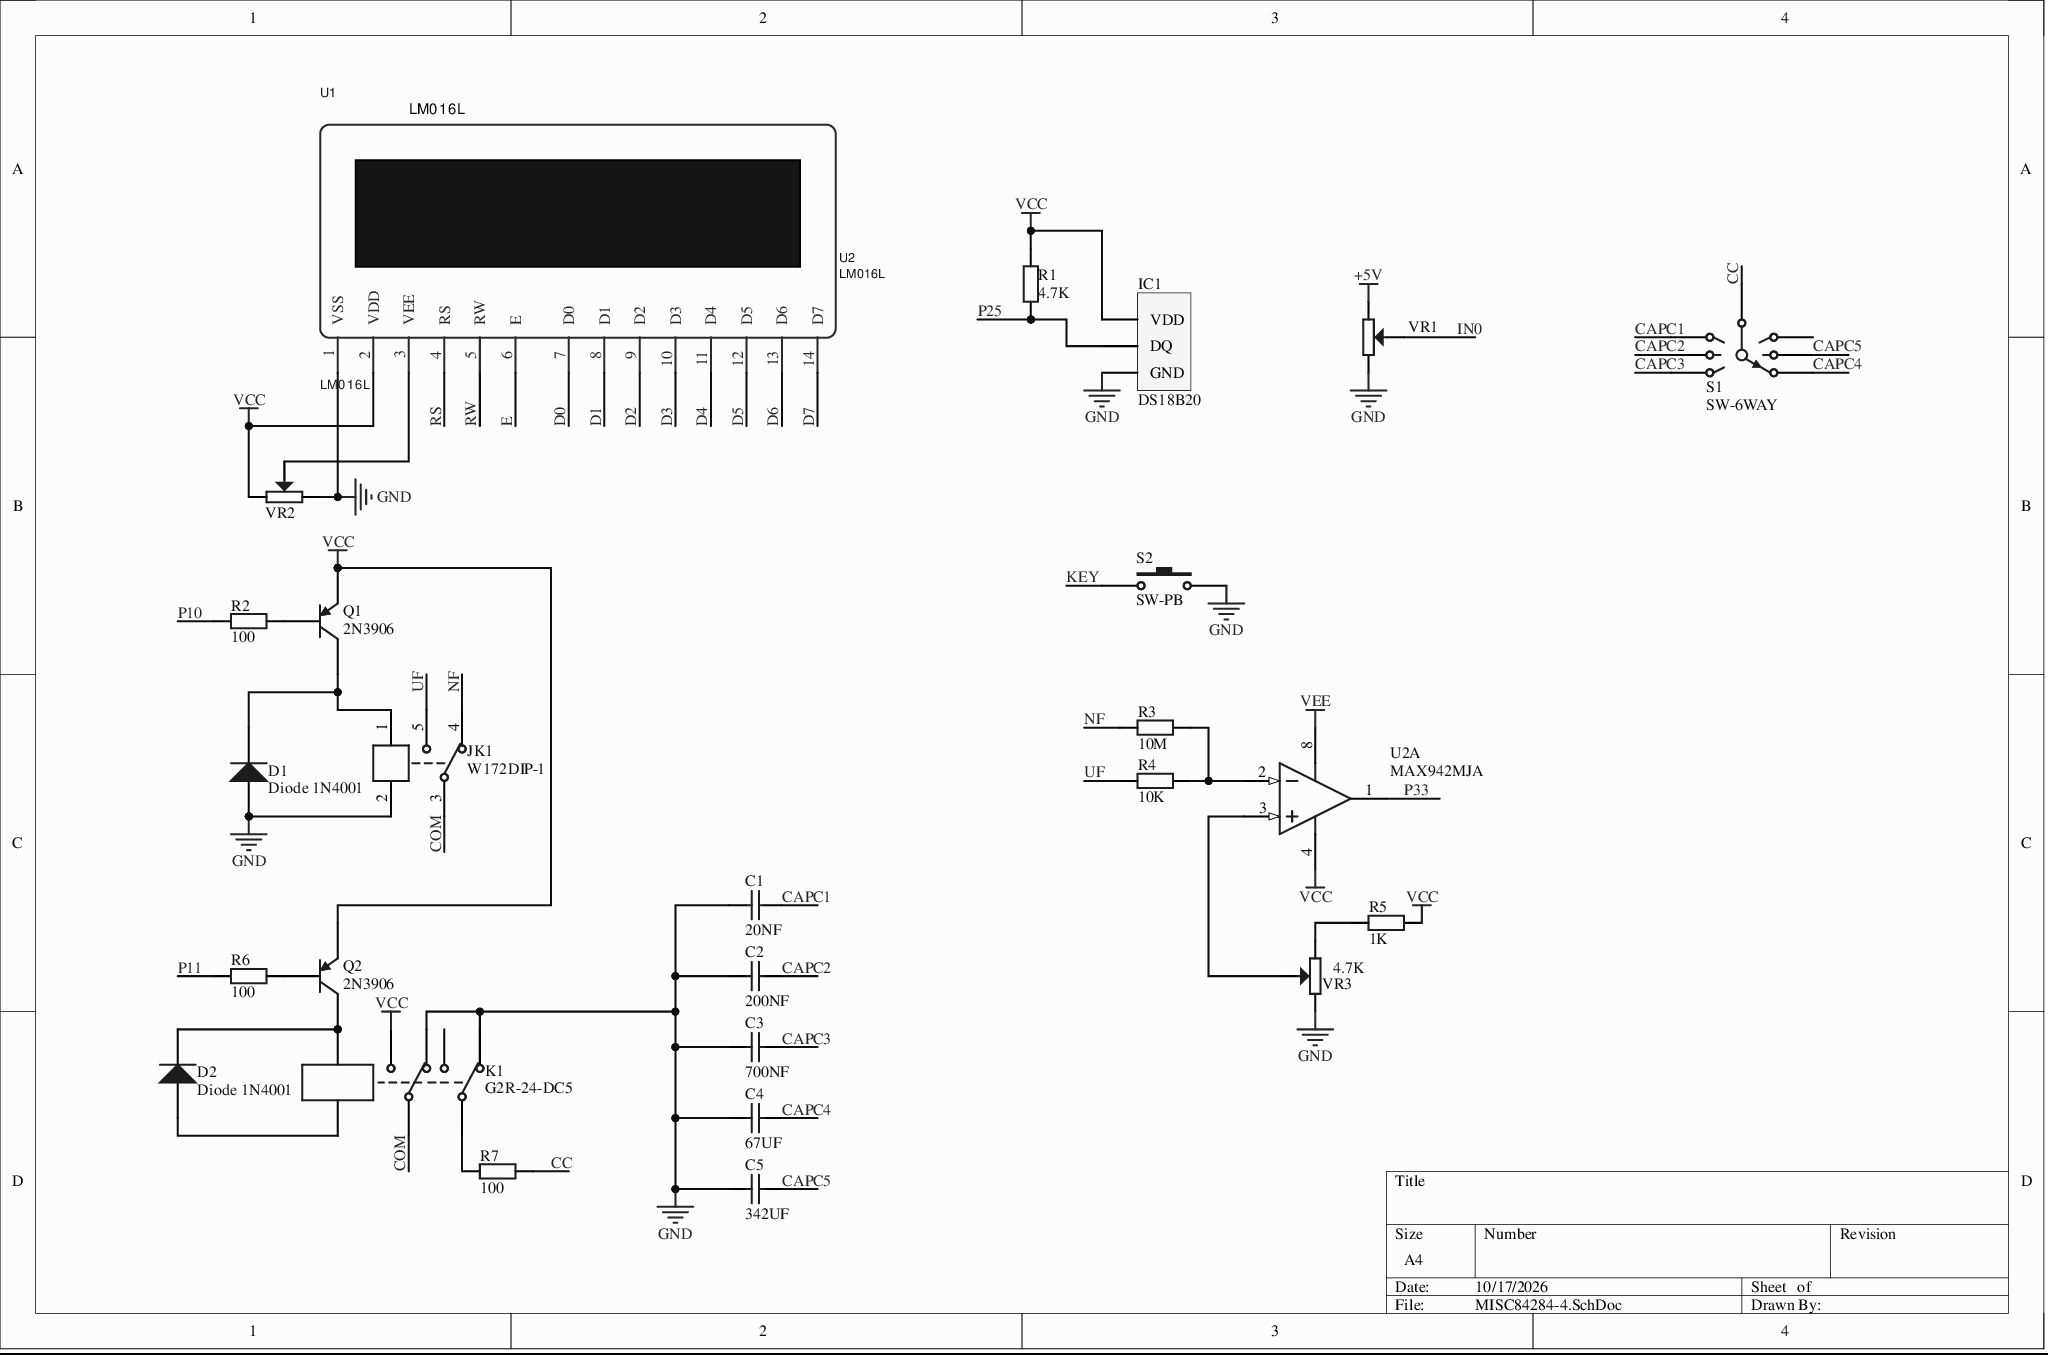
[diagram p0: MISC84284-4.SchDoc]
# Altium project MISC84284-2.PrjPcb
2 sheets, 40 parts. Net scope: global (net labels, ports and power ports of the same name join across sheets).
Board file: MISC84284.PcbDoc
Sheets:
  MISC84284-4.SchDoc
  MISC84284-5.SchDoc

## Sheet MISC84284-4.SchDoc
size A4

### Parts
C1  20NF  [RAD-0.2]
C2  200NF  [RAD-0.2]
C3  700NF  [RAD-0.2]
C4  67UF  [RAD-0.2]
C5  342UF  [RAD-0.2]
D1  Diode 1N4001  [DO-41]
D2  Diode 1N4001  [DO-41]
IC1  DS18B20  [HDR1X3]
JK1  W172DIP-1  [SRD-C_BK]
K1  G2R-24-DC5  [DIP-P8]
Q1  2N3906  [TO-92A]
Q2  2N3906  [TO-92A]
R1  4.7K  [AXIAL-0.4]
R2  100  [AXIAL-0.4]
R3  10M  [AXIAL-0.4]
R4  10K  [AXIAL-0.4]
R5  1K  [AXIAL-0.4]
R6  100  [AXIAL-0.4]
R7  100  [AXIAL-0.4]
S1  SW-6WAY  [SW-7]
S2  SW-PB  [SPST-2]
U1  LM016L  [LM016L]
U2  MAX942MJA  [JA8]  (part A of 2)
VR1  RESVR  [3296W]  (value not drawn)
VR2  RESVR  [3296W]  (value not drawn)
VR3  4.7K  [3296W]

### Nets
+5V: VR1.1
GND: C1.1 C2.1 C3.1 C4.1 C5.1 D1.1(A) IC1.1(GND) JK1.2 K1.2 K1.5 S2.2 U1.1(VSS) VR1.2 VR2.2 VR3.1
VCC: IC1.3(VDD) K1.6 Q1.1(E) Q2.1(E) R1.2 R5.1 U1.2(VDD) U2.4(GND) VR2.1
VEE: U2.8(V+)
CAPC1: C1.2 S1.1
CAPC2: C2.2 S1.2
CAPC3: C3.2 S1.3
CAPC4: C4.2 S1.6
CAPC5: C5.2 S1.5
CC: R7.1 S1.7
COM: JK1.3 K1.4
D0: U1.7(D0)
D1: U1.8(D1)
D2: U1.9(D2)
D3: U1.10(D3)
D4: U1.11(D4)
D5: U1.12(D5)
D6: U1.13(D6)
D7: U1.14(D7)
E: U1.6(E)
IN0: VR1.2
KEY: S2.1
NF: JK1.4 R3.2
P10: R2.2
P11: R6.2
P25: IC1.2(DQ) R1.1
P33: U2.1(OUT)
RS: U1.4(RS)
RW: U1.5(RW)
UF: JK1.5 R4.2
NetD1_2: D1.2(K) JK1.1 Q1.3(C)
NetD2_1: D2.1(A) K1.7
NetD2_2: D2.2(K) K1.8 Q2.3(C)
NetK1_1: K1.1 R7.2
NetQ1_2: Q1.2(B) R2.1
NetQ2_2: Q2.2(B) R6.1
NetR3_1: R3.1 R4.1 U2.2(IN-)
NetR5_2: R5.2 VR3.2
NetU1_3: U1.3(VEE) VR2.2
NetU2_3: U2.3(IN+) VR3.2

Not connected (* = marked no-connect by the designer): K1 3; S1 4

### Library data of the parts
C1-C5 = Cap: Capacitor; Value: 100pF; Published: 8-Jun-2000; LatestRevisionDate: 17-Jul-2002; LatestRevisionNote: Re-released for DXP Platform.; PackageReference: RAD-0.3; PackageDescription: Radial Cap, Thru-Hole; 2 Leads; 0.3 in Pin Spacing; Publisher: Altium Limited
D1 D2 = Diode 1N4001: 1 Amp General Purpose Rectifier; Published: 8-Jun-2000; LatestRevisionDate: 17-Jul-2002; LatestRevisionNote: Re-released for DXP Platform.; DatasheetVersion: 1998; PackageVersion: Aug-1999; PackageReference: DO-41; PackageDescription: Diode, Axial; Body 5.2 x 2.7 mm (LxDia. max), Lead Dia. 0.86 mm (max); Code_JEDEC: DO-204-AL; ComponentLink1Description: Manufacturer Link; ComponentLink2Description: Datasheet; ComponentLink2URL: http://www.fairchildsemi.com/ds/1N%2F1N4001.pdf; Publisher: Altium Limited
IC1 = DS18B20: Digital thermometer; BOM名称: Digital thermometer
JK1 = SRD-S-105D: 5V一组转换; BOM名称: 5V relay
K1 = Relay-DPDT: Dual-Pole Dual-Throw Relay; Published: 24-Mar-1999; LatestRevisionDate: 17-Jul-2002; LatestRevisionNote: Re-released for DXP Platform.; PackageReference: DIP-P8; PackageDescription: Relay; 8 Leads; Publisher: Altium Limited
Q1 Q2 = 2N3906: PNP General Purpose Amplifier; Published: 8-Jun-2000; LatestRevisionDate: 15-Jan-2003; LatestRevisionNote: PCB Footprint 'BCY-W3/D4.7' replaced; DatasheetVersion: 1997; PackageVersion: Sep-1998; PackageReference: TO-92A; PackageDescription: TO, Flat Index; 3 In-Line, Axial Leads; Body Dia. 4.5mm; Leads 0.51 x 0.48 mm (max); ComponentLink1Description: Manufacturer Link; ComponentLink2Description: Datasheet; ComponentLink2URL: http://www.fairchildsemi.com/ds/2N%2F2N3906.pdf; Publisher: Altium Limited
R1-R4 R6 R7 = Res2: Resistor; Value: 1K; Published: 8-Jun-2000; LatestRevisionDate: 17-Jul-2002; LatestRevisionNote: Re-released for DXP Platform.; PackageReference: AXIAL-0.4; PackageDescription: Axial Device, Thru-Hole; 2 Leads; 0.4 in Pin Spacing; Publisher: Altium Limited
R5 = Res2: Resistor; Published: 8-Jun-2000; LatestRevisionDate: 17-Jul-2002; LatestRevisionNote: Re-released for DXP Platform.; PackageReference: AXIAL-0.4; PackageDescription: Axial Device, Thru-Hole; 2 Leads; 0.4 in Pin Spacing; Value: 1K; Publisher: Altium Limited
S1 = SW-6WAY: 6 Way Switch; Published: 24-Mar-1999; LatestRevisionDate: 17-Jul-2002; LatestRevisionNote: Re-released for DXP Platform.; PackageReference: SW-7; PackageDescription: Switch; 7 Leads; Publisher: Altium Limited
S2 = SW-PB: Switch; Published: 24-Mar-1999; LatestRevisionDate: 17-Jul-2002; LatestRevisionNote: Re-released for DXP Platform.; PackageReference: SPST-2; PackageDescription: Switch; 2 Leads; Publisher: Altium Limited
U2 = MAX942MJA: High-speed, Low-power, 3V/5V, Rail-to-Rail Dual-Supply Comparator; Package Information: Latest Revision: 1996; Published: 16-Jan-2001; Revision: 17-Jul-2002: Re-released for DXP Platform.; Datasheet: Latest Revision: Jun-1997; Package Reference: JA8; Publisher: Altium Limited
VR3 = RESVR

## Sheet MISC84284-5.SchDoc
size A4
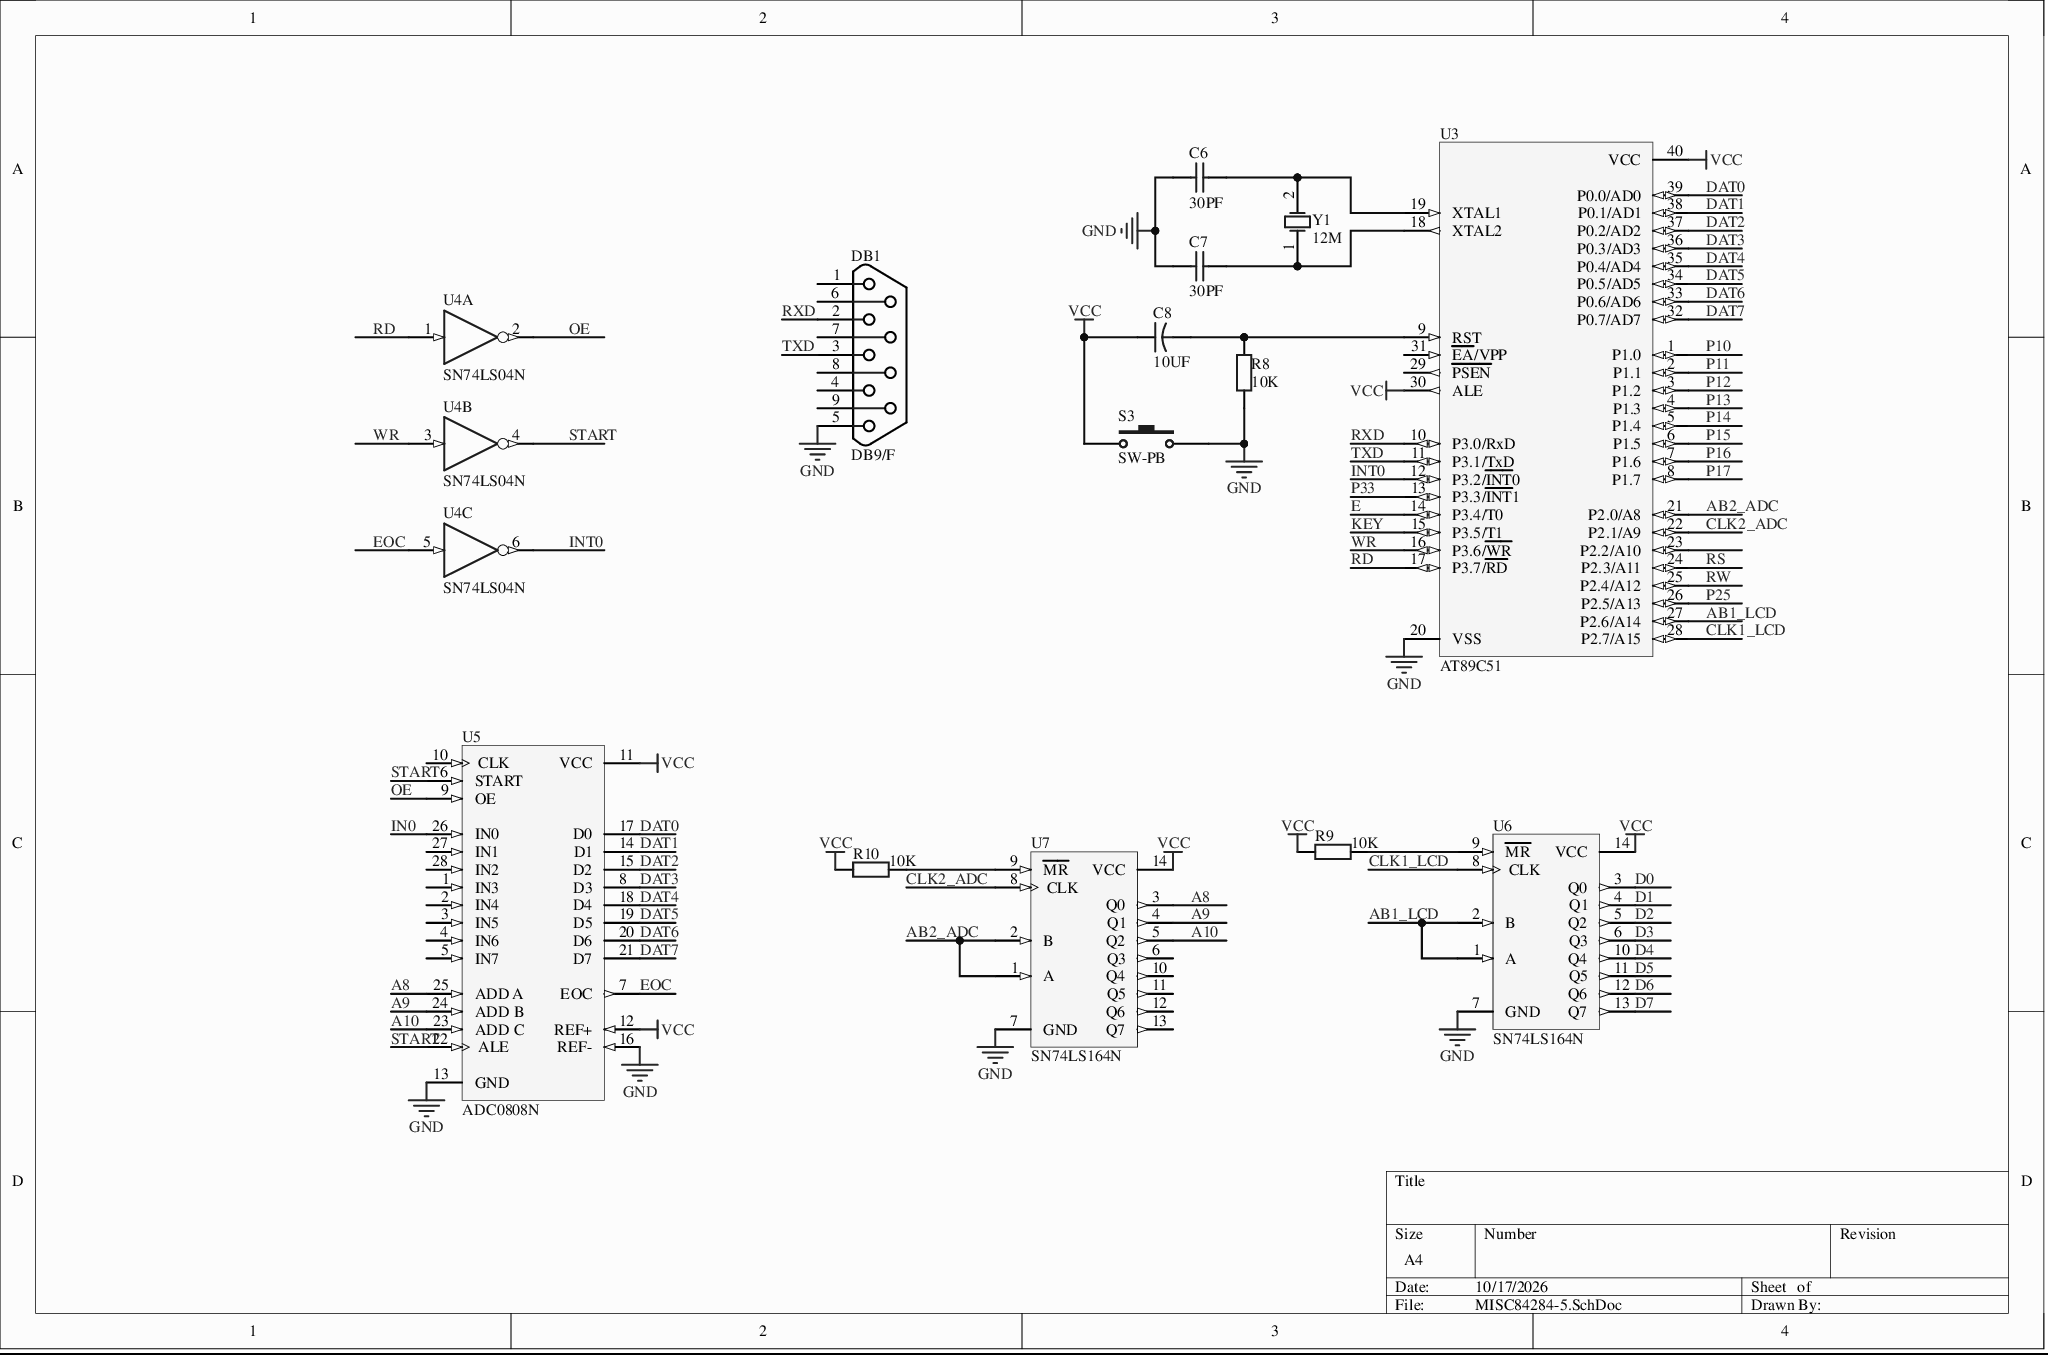
[diagram p1: MISC84284-5.SchDoc]

### Parts
C6  30PF  [RAD-0.2]
C7  30PF  [RAD-0.2]
C8  10UF  [CAPR5-4X5]
DB1  DB9/F  [DB9/F/180]
R8  10K  [AXIAL-0.4]
R9  10K  [AXIAL-0.4]
R10  10K  [AXIAL-0.4]
S3  SW-PB  [SPST-2]
U3  AT89C51  [DIP40]
U4  SN74LS04N  [646-06]  (parts A,B,C of 6)
U5  ADC0808N  [N028]
U6  SN74LS164N  [646-06]
U7  SN74LS164N  [646-06]
Y1  12M  [XTAL_US]

### Nets
GND: C6.1 C7.1 DB1.5 R8.1 S3.2 U3.20(VSS) U4.7(GND) U5.13(GND) U5.16(REF-) U6.7(GND) U7.7(GND)
VCC: C8.1 R9.2 R10.2 S3.1 U3.30(ALE) U3.40(VCC) U5.11(VCC) U5.12(REF+) U6.14(VCC) U7.14(VCC)
VDD: U4.14(VDD)
A8: U5.25(ADD_A) U7.3(Q0)
A9: U5.24(ADD_B) U7.4(Q1)
A10: U5.23(ADD_C) U7.5(Q2)
AB1_LCD: U3.27(P2.6/A14) U6.1(A) U6.2(B)
AB2_ADC: U3.21(P2.0/A8) U7.1(A) U7.2(B)
CLK1_LCD: U3.28(P2.7/A15) U6.8(CLK)
CLK2_ADC: U3.22(P2.1/A9) U7.8(CLK)
D0: U6.3(Q0)
D1: U6.4(Q1)
D2: U6.5(Q2)
D3: U6.6(Q3)
D4: U6.10(Q4)
D5: U6.11(Q5)
D6: U6.12(Q6)
D7: U6.13(Q7)
DAT0: U3.39(P0.0/AD0) U5.17(D0)
DAT1: U3.38(P0.1/AD1) U5.14(D1)
DAT2: U3.37(P0.2/AD2) U5.15(D2)
DAT3: U3.36(P0.3/AD3) U5.8(D3)
DAT4: U3.35(P0.4/AD4) U5.18(D4)
DAT5: U3.34(P0.5/AD5) U5.19(D5)
DAT6: U3.33(P0.6/AD6) U5.20(D6)
DAT7: U3.32(P0.7/AD7) U5.21(D7)
E: U3.14(P3.4/T0)
EOC: U4.5(IN) U5.7(EOC)
IN0: U5.26(IN0)
INT0: U3.12(P3.2/~{INT}0) U4.6(~{OUT})
KEY: U3.15(P3.5/T1)
OE: U4.2(~{OUT}) U5.9(OE)
P10: U3.1(P1.0)
P11: U3.2(P1.1)
P12: U3.3(P1.2)
P13: U3.4(P1.3)
P14: U3.5(P1.4)
P15: U3.6(P1.5)
P16: U3.7(P1.6)
P17: U3.8(P1.7)
P25: U3.26(P2.5/A13)
P33: U3.13(P3.3/~{INT}1)
RD: U3.17(P3.7/~{RD}) U4.1(IN)
RS: U3.24(P2.3/A11)
RW: U3.25(P2.4/A12)
RXD: DB1.2 U3.10(P3.0/RxD)
START: U4.4(~{OUT}) U5.6(START) U5.22(ALE)
TXD: DB1.3 U3.11(P3.1/TxD)
WR: U3.16(P3.6/~{WR}) U4.3(IN)
NetC6_2: C6.2 U3.19(XTAL1) Y1.2(OSC2)
NetC7_2: C7.2 U3.18(XTAL2) Y1.1(OSC1)
NetC8_2: C8.2 R8.2 U3.9(RST)
NetR9_1: R9.1 U6.9(~{MR})
NetR10_1: R10.1 U7.9(~{MR})

Not connected (* = marked no-connect by the designer): DB1 1 4 6 7 8 9; U3 23(P2.2/A10) 29(~{PSEN}) 31(~{EA}/VPP); U5 1(IN3) 2(IN4) 3(IN5) 4(IN6) 5(IN7) 10(CLK) 27(IN1) 28(IN2); U7 6(Q3) 10(Q4) 11(Q5) 12(Q6) 13(Q7)

### Library data of the parts
C6 C7 = Cap: Capacitor; Value: 100pF; Published: 8-Jun-2000; LatestRevisionDate: 17-Jul-2002; LatestRevisionNote: Re-released for DXP Platform.; PackageReference: RAD-0.3; PackageDescription: Radial Cap, Thru-Hole; 2 Leads; 0.3 in Pin Spacing; Publisher: Altium Limited
C8 = Cap2: Capacitor; Value: 100pF; Published: 23-Sep-2002; PackageReference: CAPR5-4X5; PackageDescription: Capacitor; 2 Leads; Publisher: Altium Limited
R8-R10 = Res2: Resistor; Value: 1K; Published: 8-Jun-2000; LatestRevisionDate: 17-Jul-2002; LatestRevisionNote: Re-released for DXP Platform.; PackageReference: AXIAL-0.4; PackageDescription: Axial Device, Thru-Hole; 2 Leads; 0.4 in Pin Spacing; Publisher: Altium Limited
S3 = SW-PB: Switch; Published: 24-Mar-1999; LatestRevisionDate: 17-Jul-2002; LatestRevisionNote: Re-released for DXP Platform.; PackageReference: SPST-2; PackageDescription: Switch; 2 Leads; Publisher: Altium Limited
U3 = AT89C51: 51 series MCU
U4 = SN74LS04N: Hex Inverter; Package Information: Latest Revision: 1995; Published: 15-Apr-2002; Datasheet: Latest Revision: 1999; Package Reference: 646-06; Publisher: Altium Limited
U5 = ADC0808N: CMOS Analog-to-Digital Converter with 8-Channel Multiplexer; Package Information: Latest Revision: Oct-1994; Published: 15-Apr-2002; Datasheet: Linear Circuits Data Book 1989 Volume 2 (May-1988); Package Reference: N028; Publisher: Altium Limited
U6 U7 = SN74LS164N: Serial-In Parallel-Out Shift Register; Package Information: Latest Revision: 1995; Published: 15-Apr-2002; Datasheet: Latest Revision: Dec-1999; Package Reference: 646-06; Publisher: Altium Limited
Y1 = XTAL: Crystal Oscillator; Published: 8-Jun-2000; LatestRevisionDate: 17-Jul-2002; LatestRevisionNote: Re-released for DXP Platform.; Publisher: Altium Limited

## Nets that join several sheets
GND: MISC84284-4 (15 pins), MISC84284-5 (11 pins)
VCC: MISC84284-4 (9 pins), MISC84284-5 (10 pins)
D0: MISC84284-4 (U1.7), MISC84284-5 (U6.3)
D1: MISC84284-4 (U1.8), MISC84284-5 (U6.4)
D2: MISC84284-4 (U1.9), MISC84284-5 (U6.5)
D3: MISC84284-4 (U1.10), MISC84284-5 (U6.6)
D4: MISC84284-4 (U1.11), MISC84284-5 (U6.10)
D5: MISC84284-4 (U1.12), MISC84284-5 (U6.11)
D6: MISC84284-4 (U1.13), MISC84284-5 (U6.12)
D7: MISC84284-4 (U1.14), MISC84284-5 (U6.13)
E: MISC84284-4 (U1.6), MISC84284-5 (U3.14)
IN0: MISC84284-4 (VR1.2), MISC84284-5 (U5.26)
KEY: MISC84284-4 (S2.1), MISC84284-5 (U3.15)
P10: MISC84284-4 (R2.2), MISC84284-5 (U3.1)
P11: MISC84284-4 (R6.2), MISC84284-5 (U3.2)
P25: MISC84284-4 (IC1.2 R1.1), MISC84284-5 (U3.26)
P33: MISC84284-4 (U2.1), MISC84284-5 (U3.13)
RS: MISC84284-4 (U1.4), MISC84284-5 (U3.24)
RW: MISC84284-4 (U1.5), MISC84284-5 (U3.25)